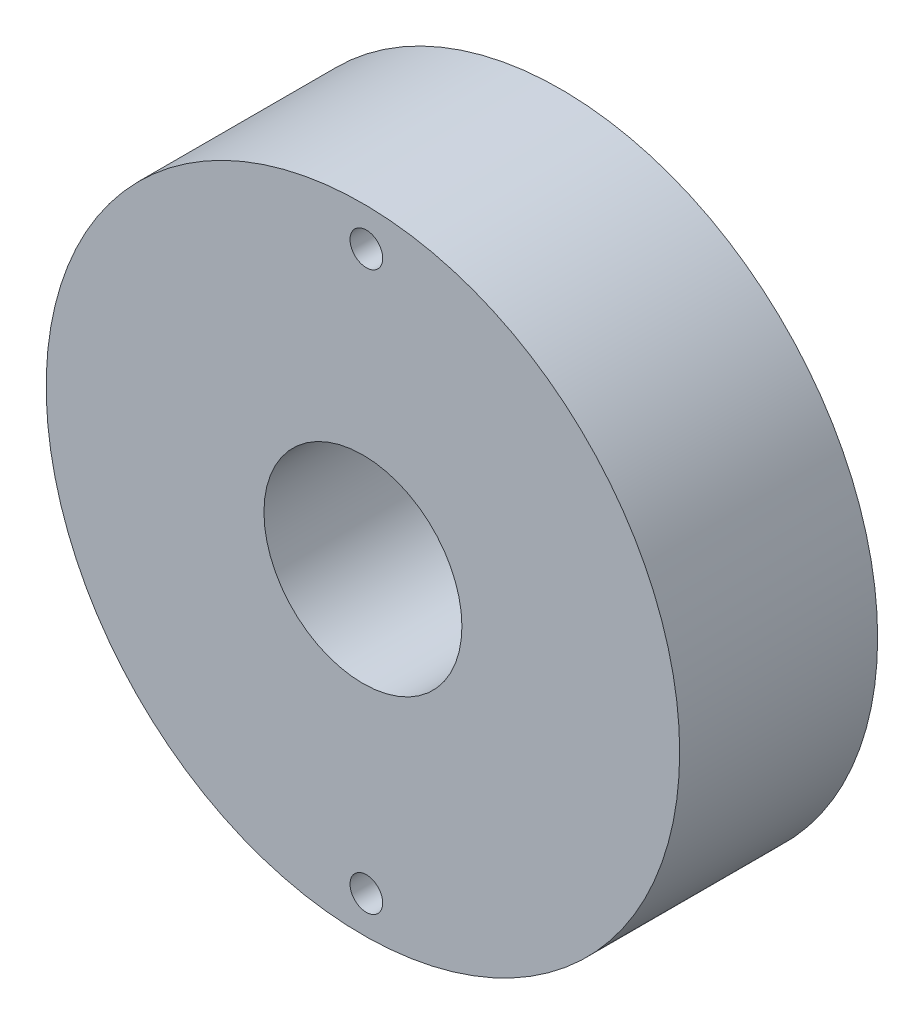
from build123d import *

# Parameters (mm, degrees)
SKETCH_1_R             = 32
SKETCH_1_R_2           = 10
EXTRUDE_1_DEPTH        = 20
HOLE_WIZARD_M4_3_D     = 3.3
HOLE_WIZARD_M4_3_DEPTH = 32.1
HOLE_WIZARD_M4_3_TIP   = 0.991420021


with BuildPart() as part:
    # 草图1 → 凸台-拉伸1 (new body)
    with BuildSketch(Plane.XY):
        with Locations((-0.347222222, 0)):
            Circle(SKETCH_1_R)
        with Locations((-0.347222222, 0)):
            Circle(SKETCH_1_R_2, mode=Mode.SUBTRACT)
    extrude(amount=EXTRUDE_1_DEPTH)

    # M4 螺纹孔3
    with Locations(Plane(origin=(0, 0, 0), x_dir=(-1, 0, 0), z_dir=(0, 0, -1))):
        with Locations((0, 28.2), (0, -28.2)):
            Hole(HOLE_WIZARD_M4_3_D / 2, depth=HOLE_WIZARD_M4_3_DEPTH)
            with Locations((0, 0, -(HOLE_WIZARD_M4_3_DEPTH + HOLE_WIZARD_M4_3_TIP / 2))):  # 118° drill point
                Cone(0, HOLE_WIZARD_M4_3_D / 2, HOLE_WIZARD_M4_3_TIP, mode=Mode.SUBTRACT)


solid = part.part
